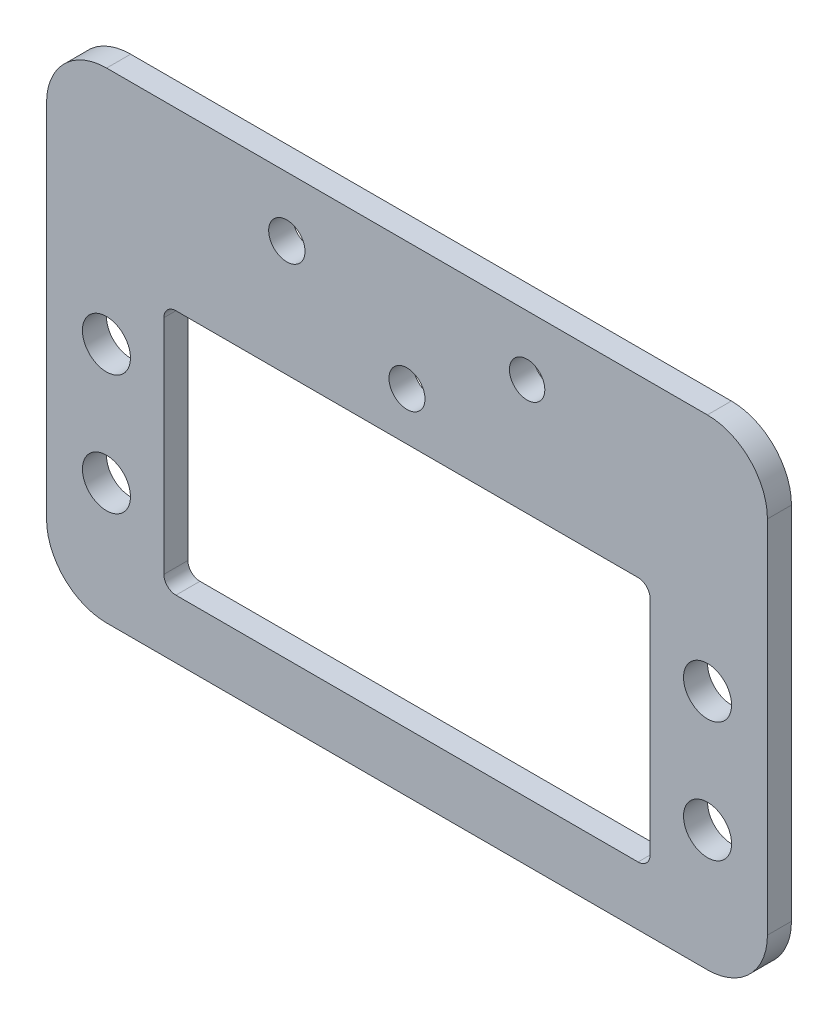
SolidWorks part; units mm, degrees
ref_plane "Front Plane" through (0, 0, 0) normal (0, 0, 1) x (1, 0, 0)
ref_plane "Top Plane" through (0, 0, 0) normal (0, 1, 0) x (1, 0, 0)
ref_plane "Right Plane" through (0, 0, 0) normal (1, 0, 0) x (0, 0, -1)
sketch "Sketch1" plane through (0, 0, 0) normal (0, 0, 1) x (1, 0, 0)
  line L1 (-22.8435, 26.4856) -> (27.1565, 26.4856)
  line L2 (-27.8435, 21.4856) -> (-27.8435, -8.5144)
  line L3 (-22.8435, -13.5144) -> (27.1565, -13.5144)
  line L4 (32.1565, 21.4856) -> (32.1565, -8.5144)
  arc A0 (27.1565, -13.5144) -> (32.1565, -8.5144) centre (27.1565, -8.5144) ccw
  arc A1 (-27.8435, -8.5144) -> (-22.8435, -13.5144) centre (-22.8435, -8.5144) ccw
  arc A2 (27.1565, 26.4856) -> (32.1565, 21.4856) centre (27.1565, 21.4856) cw
  arc A3 (-22.8435, 26.4856) -> (-27.8435, 21.4856) centre (-22.8435, 21.4856) ccw
  point P6 (32.1565, -13.5144)
  point P9 (-27.8435, -13.5144)
  point P14 (-27.8435, 26.4856)
  dimension "D3" = 5
  dimension "D1" = 60
  dimension "D2" = 40
extrude "Boss-Extrude1" add sketch "Sketch1" along normal blind 2
sketch "Sketch2" plane through (0, 0, 2) normal (0, 0, 1) x (1, 0, 0)
  line L0 (2.1565, -13.5144) -> (2.1565, 50.7332) construction
  line L1 (-22.8435, -13.5144) -> (27.1565, -13.5144) construction
  line L3 (-17.0759, 11.876) -> (21.389, 11.876)
  line L4 (-18.0759, 10.876) -> (-18.0759, -7.624)
  line L5 (-17.0759, -8.624) -> (21.389, -8.624)
  line L6 (22.389, 10.876) -> (22.389, -7.624)
  line L7 (-18.0759, 11.876) -> (22.389, -8.624) construction
  line L8 (-18.0759, -8.624) -> (22.389, 11.876) construction
  arc A0 (-18.0759, -7.624) -> (-17.0759, -8.624) centre (-17.0759, -7.624) ccw
  arc A1 (21.389, -8.624) -> (22.389, -7.624) centre (21.389, -7.624) ccw
  arc A2 (21.389, 11.876) -> (22.389, 10.876) centre (21.389, 10.876) cw
  arc A3 (-17.0759, 11.876) -> (-18.0759, 10.876) centre (-17.0759, 10.876) ccw
  point P4 (2.1565, 1.626)
  dimension "D2" = 1
  dimension "D1" = 20.5
extrude "Cut-Extrude1" cut sketch "Sketch2" against normal through all and the other way through all
sketch "Sketch3" plane through (0, 0, 2) normal (0, 0, 1) x (1, 0, 0)
  line L0 (21.389, 11.876) -> (-17.0759, 11.876) construction
  line L1 (2.1565, 11.876) -> (2.1565, 28.6699) construction
  circle A0 centre (2.1565, 15.876) radius 1.5
  circle A1 centre (12.1565, 21.526) radius 1.4721
  circle A2 centre (-7.8435, 21.526) radius 1.5125
  point P4 (2.1565, 11.876)
  dimension "D1" = 3
  dimension "D2" = 4
  dimension "D3" = 9.65
  dimension "D4" = 10
  dimension "D5" = 10
  dimension "D6" = 9.65
extrude "Cut-Extrude2" cut sketch "Sketch3" against normal through all
sketch "Sketch4" plane through (0, 0, 2) normal (0, 0, 1) x (1, 0, 0)
  line L0 (21.389, 11.876) -> (-17.0759, 11.876) construction
  line L1 (2.1565, 11.876) -> (2.1565, -24.3403) construction
  circle A0 centre (27.1717, -3.424) radius 2
  circle A1 centre (27.1717, 6.576) radius 2
  circle A2 centre (-22.8586, -3.424) radius 2
  circle A3 centre (-22.8586, 6.576) radius 2
  dimension "D1" = 10
extrude "Cut-Extrude3" cut sketch "Sketch4" against normal through all
